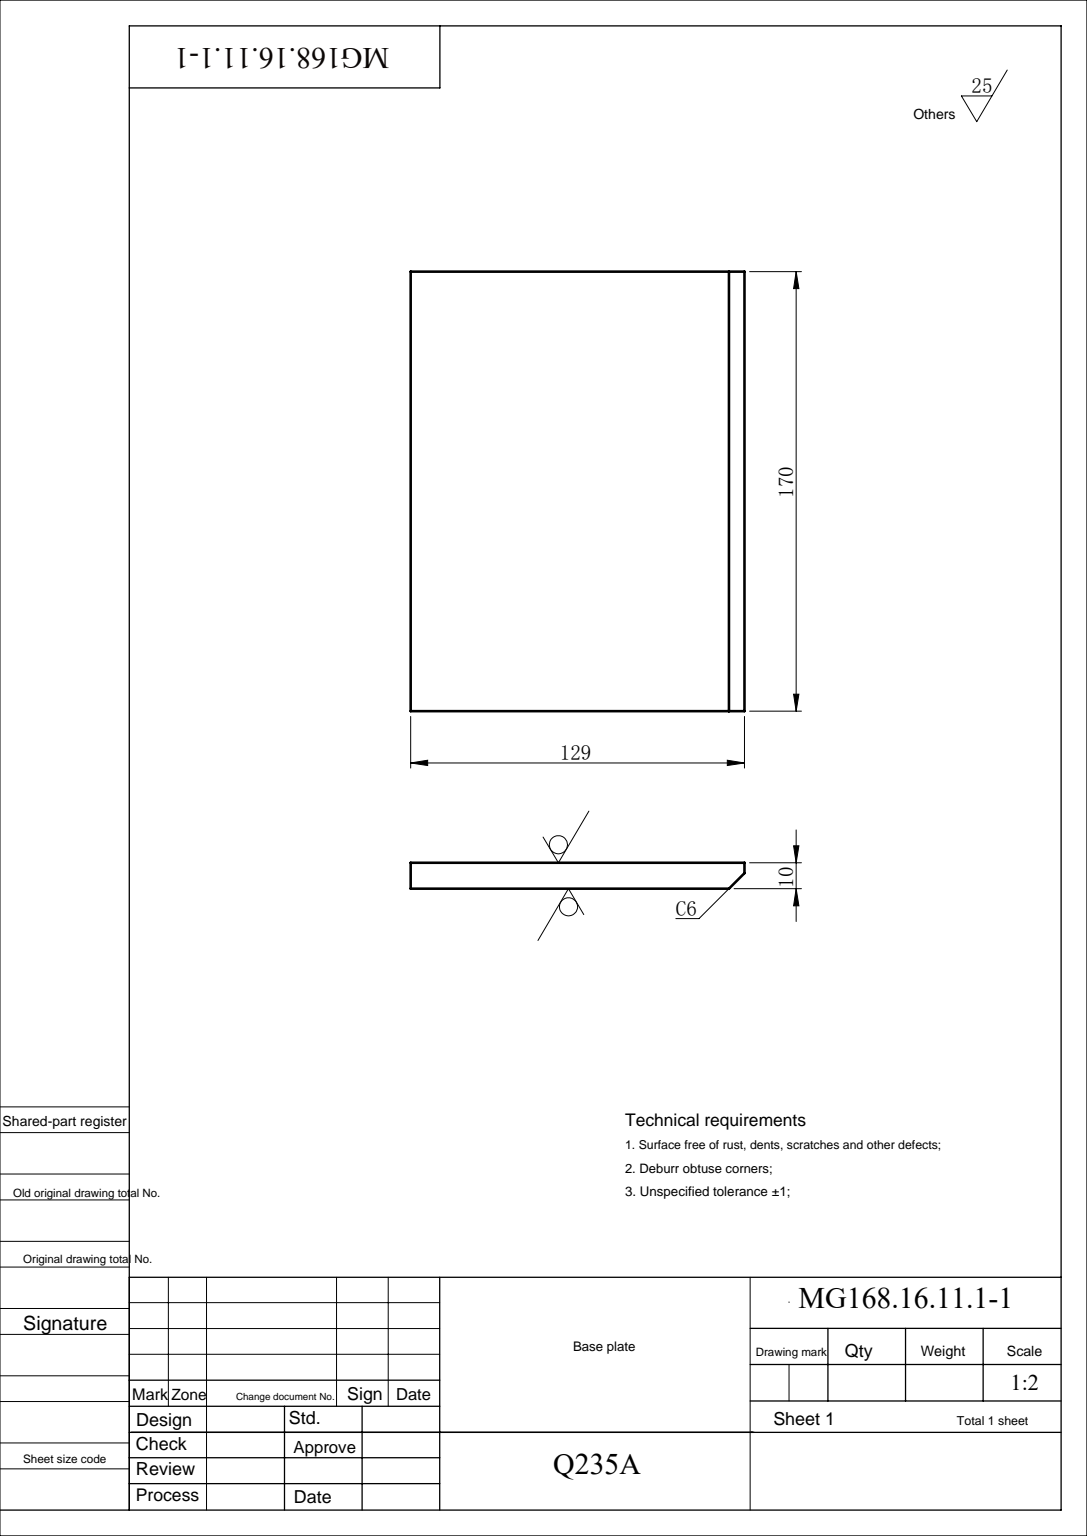
SolidWorks part; units mm, degrees
material "Q235A"
ref_plane "Front Plane" through (0, 0, 0) normal (0, 0, 1) x (1, 0, 0)
ref_plane "Top Plane" through (0, 0, 0) normal (0, 1, 0) x (1, 0, 0)
ref_plane "Right Plane" through (0, 0, 0) normal (1, 0, 0) x (0, 0, -1)
sketch "Sketch1" plane through (0, 0, 0) normal (0, 1, 0) x (1, 0, 0)
  line L0 (-97.3571, 0) -> (89.9, 0) construction
  line L1 (-58, 85) -> (71, 85)
  line L2 (-58, 85) -> (-58, -85)
  line L3 (-58, -85) -> (71, -85)
  line L4 (71, 85) -> (71, -85)
  line L5 (-50, 0) -> (50, 0) construction
  dimension "D1" = 58
  dimension "D2" = 71
  dimension "D3" = 170
extrude "Boss-Extrude1" add sketch "Sketch1" along normal mid plane 10
chamfer "Chamfer1" distance 6 angle 45 1 edges at (71, 5, 0)
